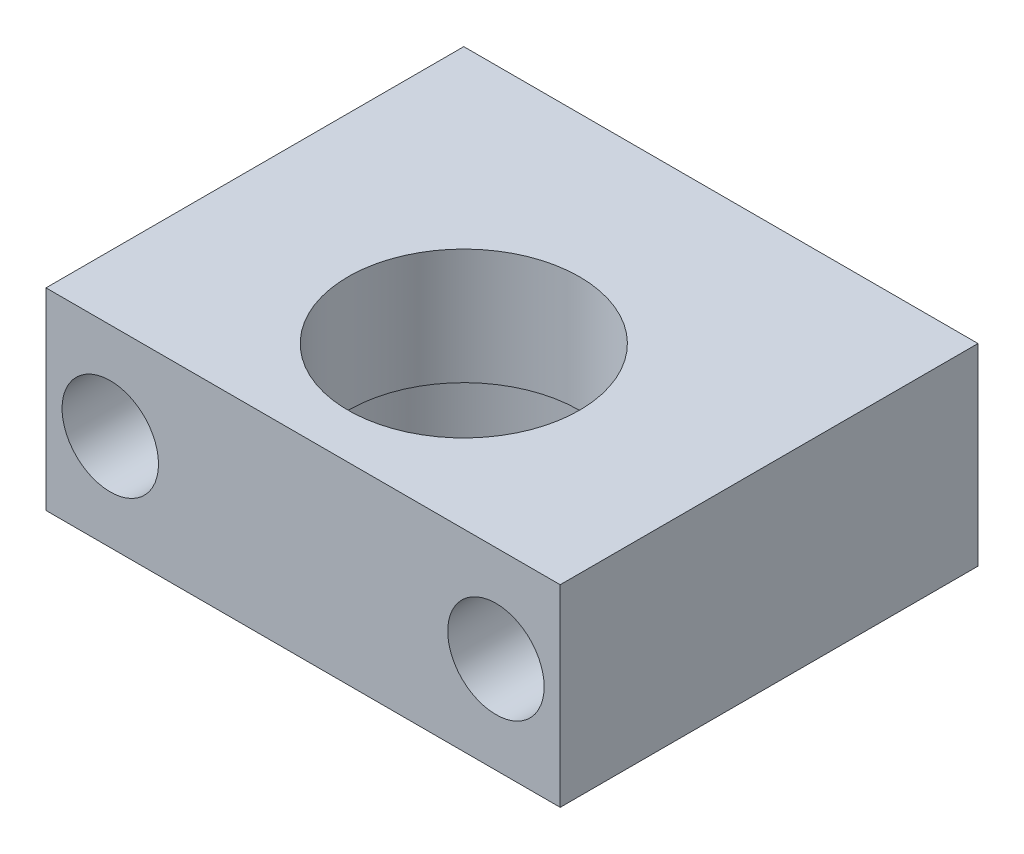
from build123d import *

# Parameters (mm, degrees)
SKETCH_1_W                  = 450
SKETCH_1_H                  = 65
EXTRUDE_1_DEPTH             = 15
CHAMFER_1_SIZE              = 2
SKETCH_2_R                  = 10
CUT_EXTRUDE_1_DEPTH         = 30
CUT_EXTRUDE_2_DEPTH         = 30
SKETCH_4_R                  = 21
CUT_EXTRUDE_3_DEPTH         = 12
SKETCH_5_R                  = 18
CUT_EXTRUDE_4_DEPTH         = 229.046596116
HOLE_WIZARD_2_D             = 6.6
HOLE_WIZARD_2_DEPTH         = 31.5
HOLE_WIZARD_2_CBORE_D       = 11
HOLE_WIZARD_2_CBORE_DEPTH   = 6.8
HOLE_WIZARD_M6_1_D          = 5
HOLE_WIZARD_2_2_D           = 9
HOLE_WIZARD_2_2_CBORE_D     = 15
HOLE_WIZARD_2_2_CBORE_DEPTH = 55
HOLE_WIZARD_M5_1_D          = 4.2
HOLE_WIZARD_M5_1_DEPTH      = 12.4
HOLE_WIZARD_M5_1_TIP        = 1.2618073
SKETCH_15_W                 = 237.437546179
SKETCH_15_H                 = 159.818796437
CUT_EXTRUDE_6_DEPTH         = 230.306018238


with BuildPart() as part:
    # 草图1 → 凸台-拉伸1 (new, symmetric)
    with BuildSketch(Plane(origin=(0, 0, 0), x_dir=(1, 0, 0), z_dir=(0, 1, 0))):
        Rectangle(SKETCH_1_W, SKETCH_1_H)
    extrude(amount=EXTRUDE_1_DEPTH, both=True)

    # 倒角1
    chamfer_1_edges = [part.edges().sort_by_distance(p)[0] for p in [
        (225, 0, 32.5),
        (-225, 0, 32.5),
    ]]
    chamfer(chamfer_1_edges, length=CHAMFER_1_SIZE)

    # 草图2 → 切除-拉伸1 (cut)
    with BuildSketch(Plane(origin=(0, 15, 0), x_dir=(1, 0, 0), z_dir=(0, 1, 0))):
        with Locations(Location((-200, 0, 0), (0, 0, 270))):
            Circle(SKETCH_2_R)
        with Locations(Location((200, 0, 0), (0, 0, 90))):
            Circle(SKETCH_2_R)
    extrude(amount=-CUT_EXTRUDE_1_DEPTH, mode=Mode.SUBTRACT)

    # 草图3 → 切除-拉伸2 (cut)
    with BuildSketch(Plane(origin=(0, 15, 0), x_dir=(1, 0, 0), z_dir=(0, 1, 0))):
        with BuildLine():
            Line((-225, 1), (-182, 1))
            ThreePointArc((-182, 1), (-181, 0), (-182, -1))
            Line((-182, -1), (-225, -1))
            ThreePointArc((-225, -1), (-226, 0), (-225, 1))
        make_face()
        with BuildLine():
            Line((225, 1), (182, 1))
            ThreePointArc((182, 1), (181, 0), (182, -1))
            Line((182, -1), (225, -1))
            ThreePointArc((225, -1), (226, 0), (225, 1))
        make_face()
    extrude(amount=-CUT_EXTRUDE_2_DEPTH, mode=Mode.SUBTRACT)

    # 草图4 → 切除-拉伸3 (cut)
    with BuildSketch(Plane(origin=(0, -15, 0), x_dir=(1, 0, 0), z_dir=(0, 1, 0))):
        with Locations(Location((0, -7.5, 0), (0, 0, 270))):
            Circle(SKETCH_4_R)
    extrude(amount=CUT_EXTRUDE_3_DEPTH, mode=Mode.SUBTRACT)

    # 草图5 → 切除-拉伸4 (cut, through all)
    with BuildSketch(Plane(origin=(0, -3, 0), x_dir=(-1, 0, 0), z_dir=(0, -1, 0))):
        with Locations(Location((0, -7.5, 0), (0, 0, 90))):
            Circle(SKETCH_5_R)
    extrude(amount=-CUT_EXTRUDE_4_DEPTH, mode=Mode.SUBTRACT)

    # Hole Wizard 2
    with Locations(Plane.XY.offset(32.5)):
        with Locations((215, -7.5), (215, 7.5), (-215, 7.5), (-215, -7.5)):
            CounterBoreHole(HOLE_WIZARD_2_D / 2, HOLE_WIZARD_2_CBORE_D / 2, HOLE_WIZARD_2_CBORE_DEPTH, depth=HOLE_WIZARD_2_DEPTH)

    # M6 螺纹孔1 (through all)
    with Locations(Plane.XY.offset(-1)):
        with Locations((215, -7.5), (215, 7.5), (-215, -7.5), (-215, 7.5)):
            Hole(HOLE_WIZARD_M6_1_D / 2)

    # Hole Wizard 2 2 (through all)
    with Locations(Plane.XY.offset(32.5)):
        with Locations((150, 0), (30, 0), (-30, 0), (-150, 0)):
            CounterBoreHole(HOLE_WIZARD_2_2_D / 2, HOLE_WIZARD_2_2_CBORE_D / 2, HOLE_WIZARD_2_2_CBORE_DEPTH)

    # M5 螺纹孔1
    with Locations(Plane(origin=(0, -15, 0), x_dir=(-1, 0, 0), z_dir=(0, -1, 0))):
        with Locations((-17.324116139, 9.824116139), (17.324116139, 9.824116139), (17.324116139, -24.824116139), (-17.324116139, -24.824116139)):
            Hole(HOLE_WIZARD_M5_1_D / 2, depth=HOLE_WIZARD_M5_1_DEPTH)
            with Locations((0, 0, -(HOLE_WIZARD_M5_1_DEPTH + HOLE_WIZARD_M5_1_TIP / 2))):  # 118° drill point
                Cone(0, HOLE_WIZARD_M5_1_D / 2, HOLE_WIZARD_M5_1_TIP, mode=Mode.SUBTRACT)

    # 草图15 → 切除-拉伸6 (cut, through all)
    with BuildSketch(Plane.XZ.offset(15)):
        with Locations((158.71877309, 13.745723836)):
            Rectangle(SKETCH_15_W, SKETCH_15_H)
        with Locations((-158.71877309, 13.745723836)):
            Rectangle(SKETCH_15_W, SKETCH_15_H)
    extrude(amount=-CUT_EXTRUDE_6_DEPTH, mode=Mode.SUBTRACT)


solid = part.part
